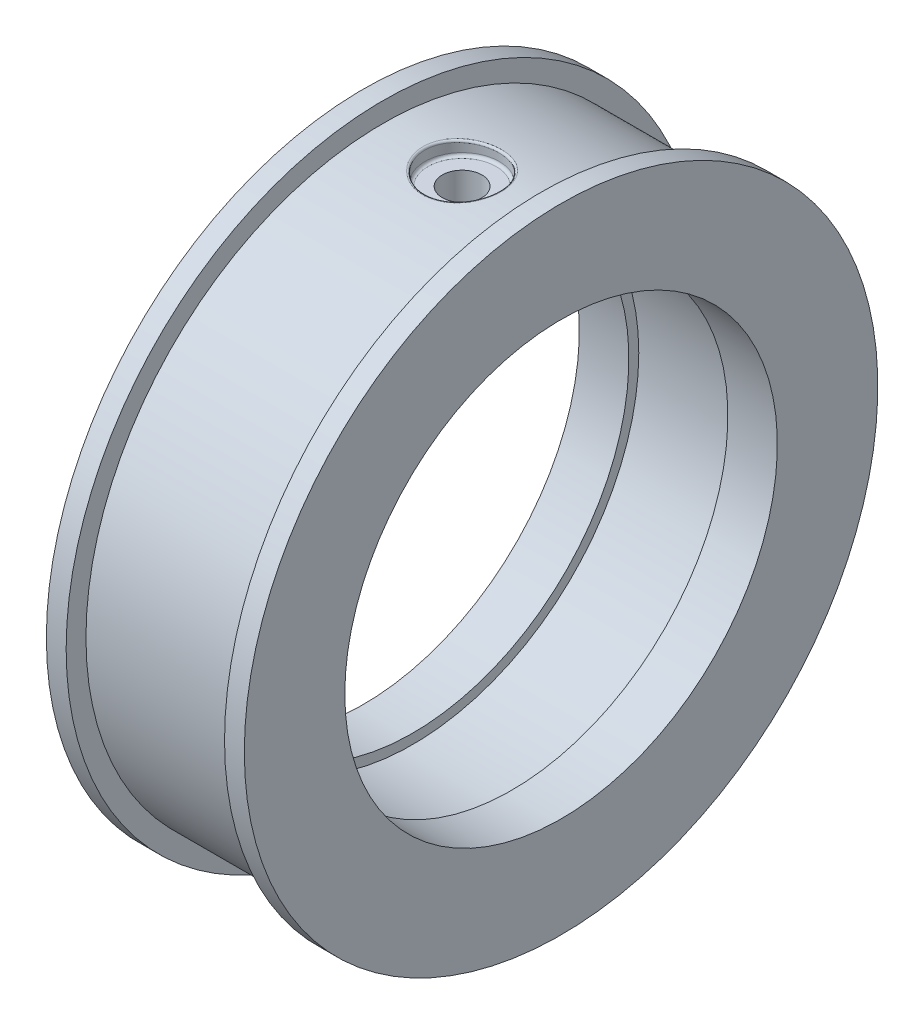
SolidWorks part; units mm, degrees
ref_plane "Front Plane" through (0, 0, 0) normal (0, 0, 1) x (1, 0, 0)
ref_plane "Top Plane" through (0, 0, 0) normal (0, 1, 0) x (1, 0, 0)
ref_plane "Right Plane" through (0, 0, 0) normal (1, 0, 0) x (0, 0, -1)
sketch "Sketch1" plane through (0, 0, 0) normal (0, 0, 1) x (1, 0, 0)
  line L0 (-19.0368, 0) -> (19.2228, 0) construction
  line L1 (-8.3897, 21.85) -> (-8.3897, 32)
  line L2 (-8.3897, 32) -> (-6.3897, 32)
  line L3 (-6.3897, 32) -> (-6.3897, 30)
  line L4 (-6.3897, 30) -> (9.6103, 30)
  line L5 (9.6103, 30) -> (9.6103, 32)
  line L6 (9.6103, 32) -> (11.6103, 32)
  line L7 (11.6103, 32) -> (11.6103, 21.85)
  line L8 (11.6103, 21.85) -> (6.6103, 21.85)
  line L9 (6.6103, 21.85) -> (6.6103, 22.85)
  line L10 (6.6103, 22.85) -> (-3.3897, 22.85)
  line L11 (-3.3897, 22.85) -> (-3.3897, 21.85)
  line L12 (-3.3897, 21.85) -> (-8.3897, 21.85)
  dimension "D2" = 20
  dimension "D3" = 16
  dimension "D4" = 2
  dimension "D5" = 21.85
  dimension "D6" = 21.85
  dimension "D7" = 22.85
  dimension "D8" = 10
  dimension "D9" = 5
  dimension "D10" = 30
  dimension "D11" = 32
  dimension "D12" = 32
revolve "Revolve1" add sketch "Sketch1" angle 360 about L0
ref_plane "Plane1" through (0, 30, 0) normal (0, 1, 0) x (1, 0, 0)
sketch "Sketch2" plane through (0, 30, 0) normal (0, 1, 0) x (1, 0, 0)
  line L0 (-6.3897, 0) -> (9.6103, 0)
  line L1 (-6.3897, -32) -> (-6.3897, 32) construction
  line L2 (9.6103, 30) -> (9.6103, -30) construction
hole_wizard "Hole1" positions "Sketch3" profile "Sketch4" legacy
sketch "Sketch3" plane through (0, 30, 0) normal (0, 1, 0) x (1, 0, 0)
  line L0 (-6.3897, 0) -> (9.6103, 0) construction
  point P0 (1.6103, 0)
sketch "Sketch4" plane through (1.6103, 30, 0) normal (1, 0, 0) x (0, 0, 1)
  line L0 (0, 0) -> (0, 1.5)
  line L1 (0, 1.5) -> (3.75, 1.5)
  line L2 (3.75, 1.5) -> (3.75, 0)
  line L3 (3.75, 0) -> (0, 0)
  line L4 (0, 110) -> (0, -10) construction
  dimension "直径" = 7.5
  dimension "深度" = 1.5
hole_wizard "Hole2" positions "Sketch5" profile "Sketch6" legacy
sketch "Sketch5" plane through (0, 28.5, 0) normal (0, 1, 0) x (1, 0, 0)
  point P0 (1.6103, 0)
sketch "Sketch6" plane through (1.6103, 28.5, 0) normal (1, 0, 0) x (0, 0, 1)
  line L0 (0, 0) -> (0, 5.65)
  line L1 (0, 5.65) -> (2, 5.65)
  line L2 (2, 5.65) -> (2, 0)
  line L3 (2, 0) -> (0, 0)
  line L4 (0, 110) -> (0, -10) construction
  dimension "直径" = 4
  dimension "深度" = 5.65
ref_plane "Plane2" through (0, -30, 0) normal (0, -1, 0) x (-1, 0, 0)
sketch "Sketch8" plane through (0, -30, 0) normal (0, -1, 0) x (-1, 0, 0)
  line L0 (6.3897, 0) -> (-9.6103, 0) construction
  line L1 (6.3897, 0) -> (-9.6103, 0)
hole_wizard "Dowel Hole1" positions "Sketch9" profile "Sketch10" hole size "Ø4.0" standard "GB"
sketch "Sketch9" plane through (0, -30, 0) normal (0, -1, 0) x (-1, 0, 0)
  line L0 (6.3897, 0) -> (-9.6103, 0) construction
  point P0 (-1.6103, 0)
sketch "Sketch10" plane through (1.6103, -30, 0) normal (1, 0, 0) x (0, 0, -1)
  line L0 (0, 0) -> (0, 5.2017)
  line L1 (0, 5.2017) -> (2, 4)
  line L2 (2, 4) -> (2, 0)
  line L5 (2, 0) -> (0, 0)
  line L10 (0, 5.2017) -> (-2, 4) construction
  line L11 (0, -6.35) -> (0, 107.95) construction
  dimension "孔直径" = 4
  dimension "孔深度" = 4
  dimension "导头角度" = 118
fillet "Fillet1" radius 0.2 1 edges at (2.44, 29.7763, -3.6571)
fillet "Fillet2" radius 0.3 1 edges at (1.6103, 28.5, 3.75)
